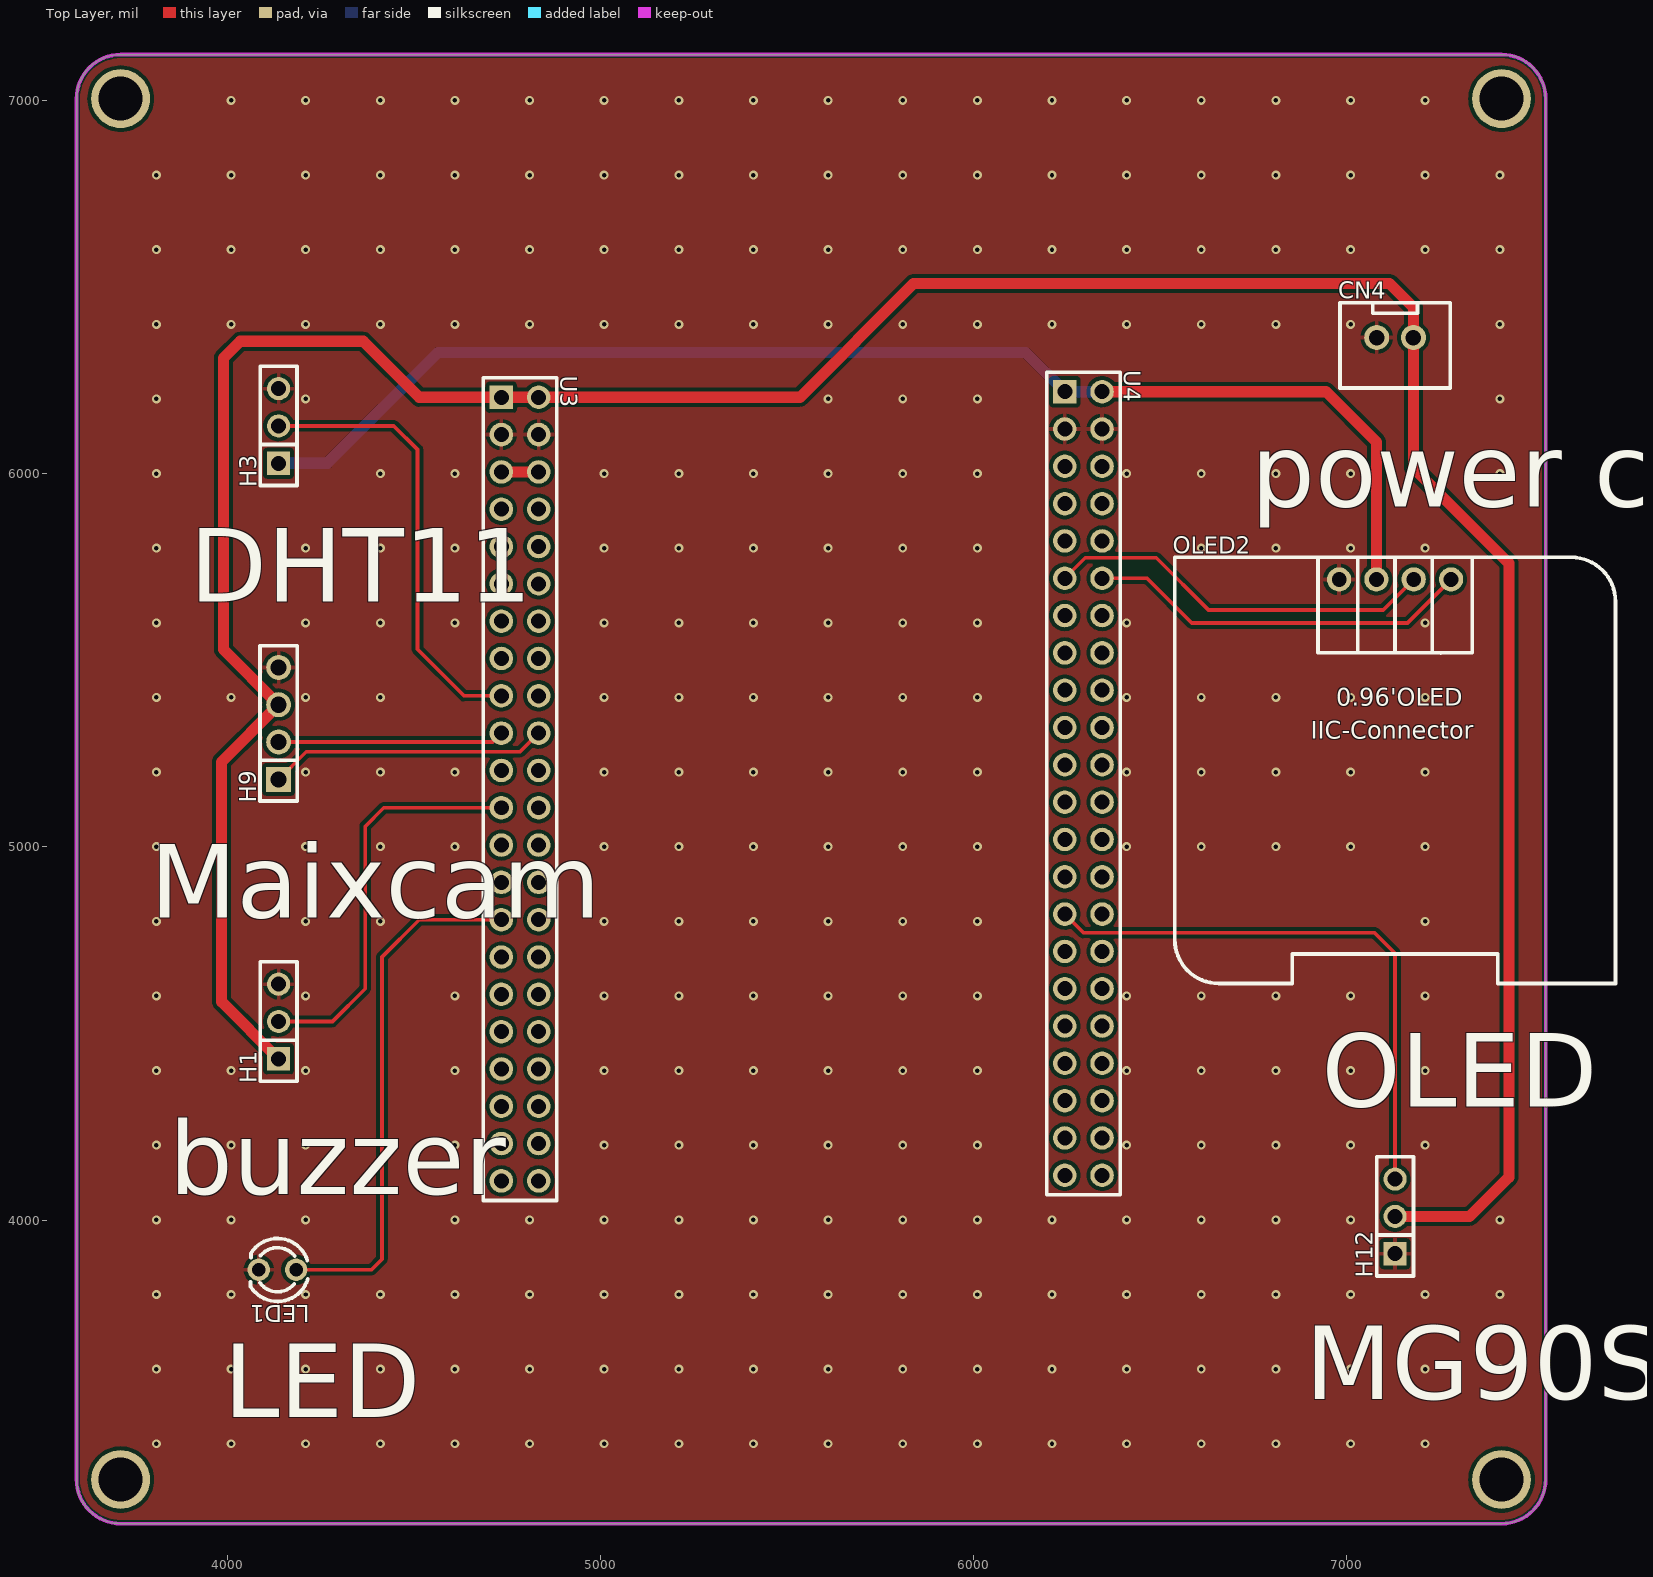
[diagram p0: Top Layer view]
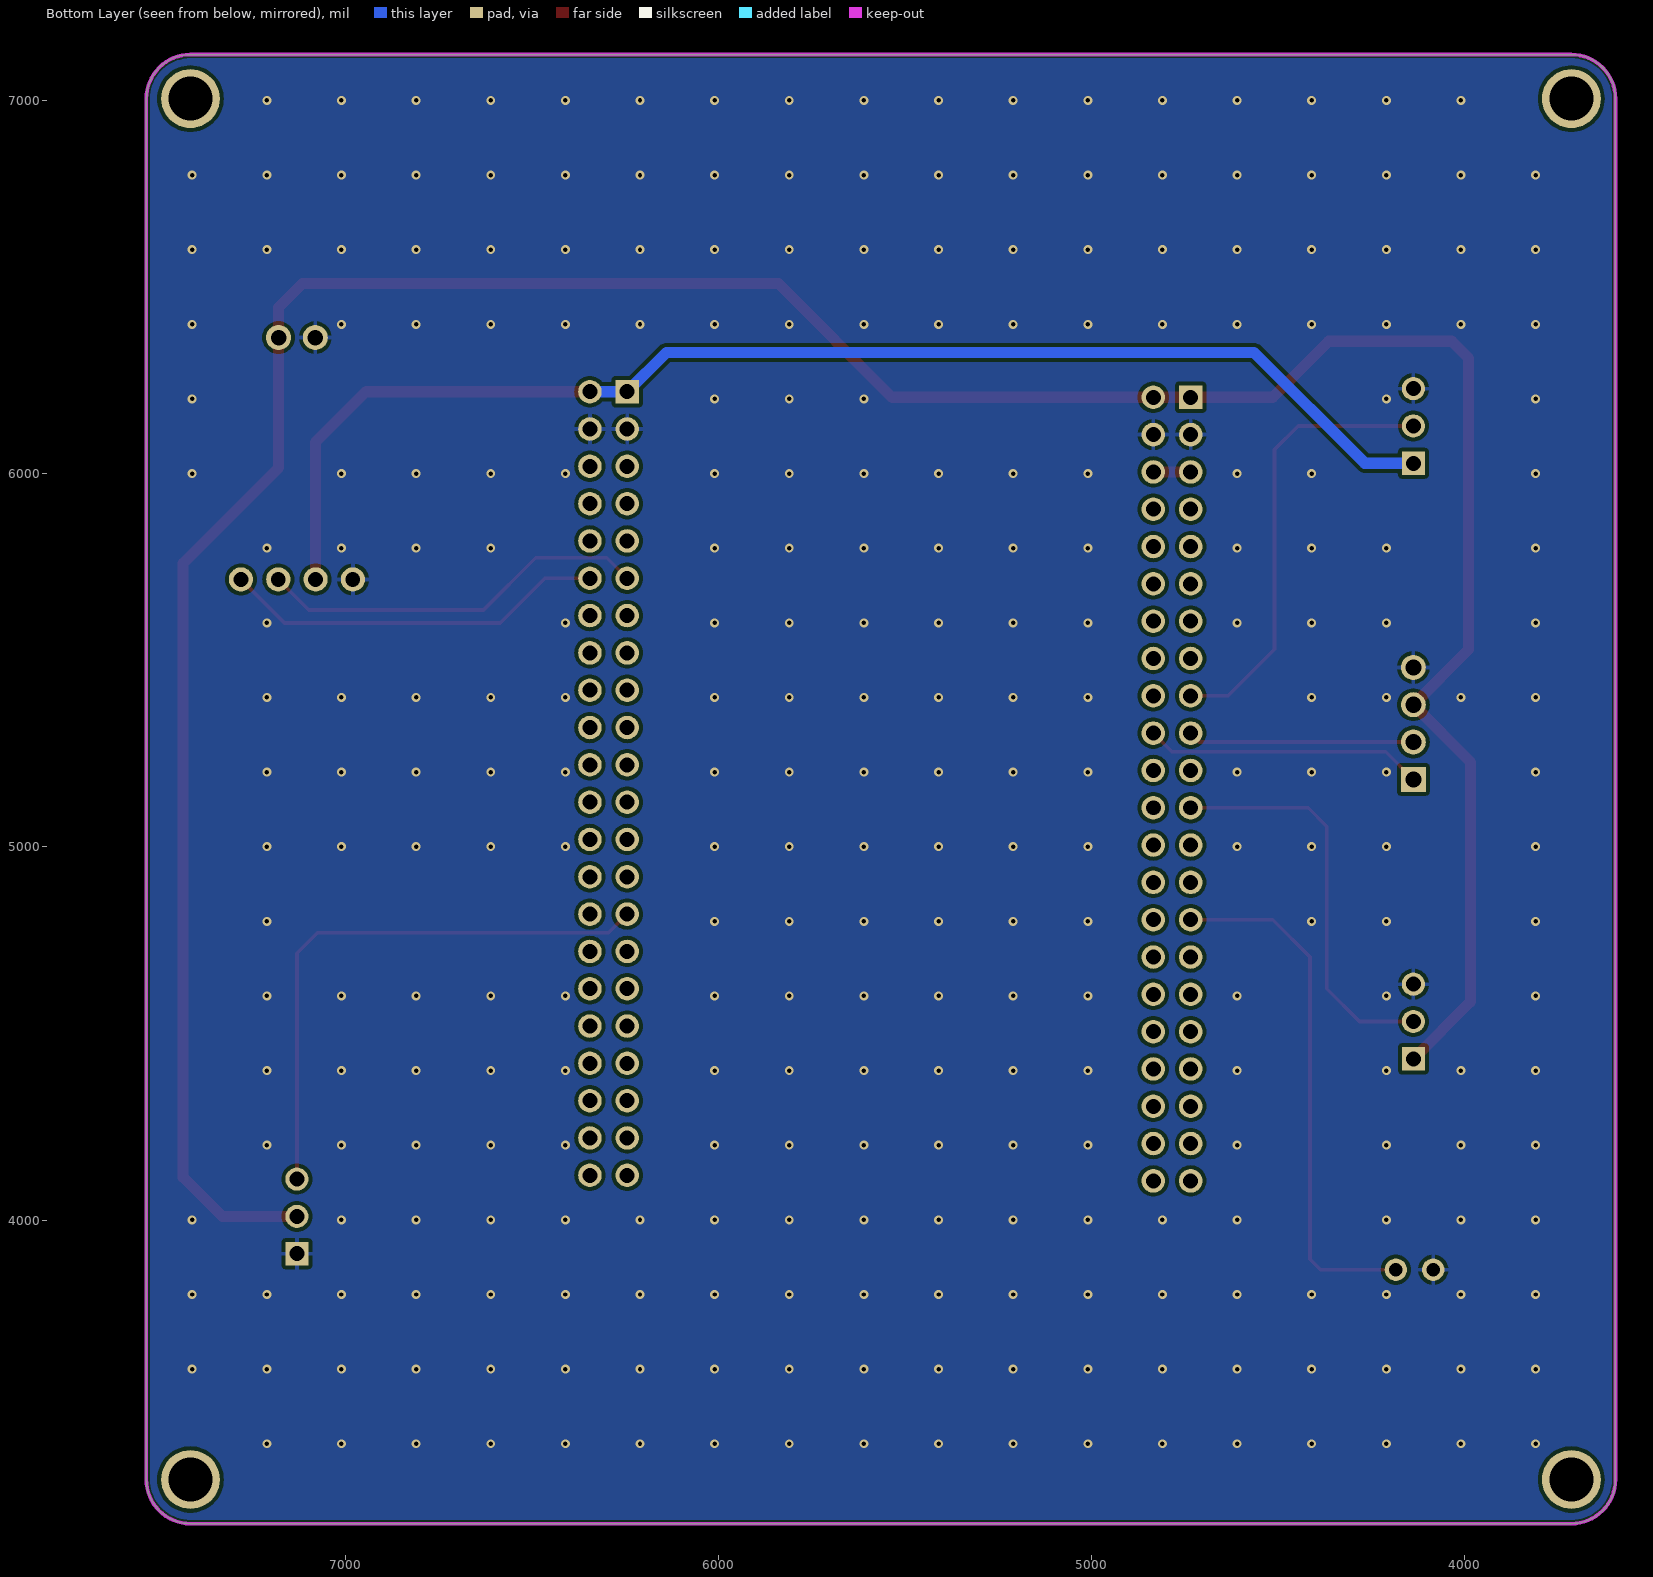
[diagram p1: Bottom Layer view, seen from below]
# Altium PCB MISC89054.pcbdoc
Units mil, origin at the board's own origin, x right, y up, seen from the top; angles counter-clockwise.
Board outline 3937.01 x 3937.01 mil, 2 copper layers (Top Layer, Bottom Layer), stack 62.206 mil thick; 9 components, 82 nets, 113 pads, 291 vias.

## Layer stack, top to bottom
Top Solder Mask Layer: solder mask 0.394, Dk 3.3
Top Layer: signal copper 1.379
Dielectric1: surface 59.449, FR4, Dk 4.5
Bottom Layer: signal copper 1.378
Bottom Solder Mask Layer: solder mask 0.394, Dk 3.3

## Board outline
3714.61,7123.5 ccw(c3714.61,7005.39) 3596.5,7005.39 3596.5,3304.61 ccw(c3714.61,3304.61) 3714.61,3186.5 7415.39,3186.5 ccw(c7415.39,3304.61) 7533.5,3304.61 7533.5,7005.39 ccw(c7415.39,7005.39) 7415.39,7123.5 3714.61,7123.5

## Design rules (kind name [scope] priority, off if disabled: settings)
BoardOutlineClearance copperThickness2oz_1 [All] p2 off: genericclearance=7.99 ignorepadtopadclearanceinfootprint=FALSE except(0: Arc-SplitContinuation Track-SplitContinuation SMDPad-SplitContinuation THPad-SplitContinuation Via-SplitContinuation Fill-SplitContinuation Region-SplitContinuation Poly-SplitContinuation Text-SplitContinuation Hole-SplitContinuation; 5.98: Arc-CutoutEdge Track-CutoutEdge SMDPad-CutoutEdge THPad-CutoutEdge Via-CutoutEdge Text-CutoutEdge; 6.9: Hole-OutlineEdge Hole-CutoutEdge; 10: Poly-OutlineEdge Poly-CutoutEdge; 11.81: Arc-OutlineEdge Track-OutlineEdge SMDPad-OutlineEdge THPad-OutlineEdge Via-OutlineEdge Fill-OutlineEdge Region-OutlineEdge Text-OutlineEdge Fill-CutoutEdge Region-CutoutEdge)
BoardOutlineClearance Plane_innerPlane_1 [All] p4 off: genericclearance=4.02 ignorepadtopadclearanceinfootprint=FALSE except(0: Arc-SplitContinuation Track-SplitContinuation SMDPad-SplitContinuation THPad-SplitContinuation Via-SplitContinuation Fill-SplitContinuation Region-SplitContinuation Poly-SplitContinuation Text-SplitContinuation Hole-SplitContinuation; 5.98: Arc-CutoutEdge Track-CutoutEdge SMDPad-CutoutEdge THPad-CutoutEdge Via-CutoutEdge Text-CutoutEdge; 6.9: Hole-OutlineEdge Hole-CutoutEdge; 10: Poly-OutlineEdge Poly-CutoutEdge; 11.81: Arc-OutlineEdge Track-OutlineEdge SMDPad-OutlineEdge THPad-OutlineEdge Via-OutlineEdge Fill-OutlineEdge Region-OutlineEdge Text-OutlineEdge Fill-CutoutEdge Region-CutoutEdge)
BoardOutlineClearance Copper_copperRegion_1 [All] p6 off: genericclearance=4.02 ignorepadtopadclearanceinfootprint=FALSE except(0: Arc-SplitContinuation Track-SplitContinuation SMDPad-SplitContinuation THPad-SplitContinuation Via-SplitContinuation Fill-SplitContinuation Region-SplitContinuation Poly-SplitContinuation Text-SplitContinuation Hole-SplitContinuation; 5.98: Arc-CutoutEdge Track-CutoutEdge SMDPad-CutoutEdge THPad-CutoutEdge Via-CutoutEdge Text-CutoutEdge; 6.9: Hole-OutlineEdge Hole-CutoutEdge; 10: Poly-OutlineEdge Poly-CutoutEdge; 11.81: Arc-OutlineEdge Track-OutlineEdge SMDPad-OutlineEdge THPad-OutlineEdge Via-OutlineEdge Fill-OutlineEdge Region-OutlineEdge Text-OutlineEdge Fill-CutoutEdge Region-CutoutEdge)
BoardOutlineClearance Copper_copperRegion_copperThickness1oz_1 [All] p8 off: genericclearance=4.02 ignorepadtopadclearanceinfootprint=FALSE except(0: Arc-SplitContinuation Track-SplitContinuation SMDPad-SplitContinuation THPad-SplitContinuation Via-SplitContinuation Fill-SplitContinuation Region-SplitContinuation Poly-SplitContinuation Text-SplitContinuation Hole-SplitContinuation; 5.98: Arc-CutoutEdge Track-CutoutEdge SMDPad-CutoutEdge THPad-CutoutEdge Via-CutoutEdge Text-CutoutEdge; 6.9: Hole-OutlineEdge Hole-CutoutEdge; 10: Poly-OutlineEdge Poly-CutoutEdge; 11.81: Arc-OutlineEdge Track-OutlineEdge SMDPad-OutlineEdge THPad-OutlineEdge Via-OutlineEdge Fill-OutlineEdge Region-OutlineEdge Text-OutlineEdge Fill-CutoutEdge Region-CutoutEdge)
BoardOutlineClearance Copper_copperRegion_Copper_copperRegion_1 [All] p10 off: genericclearance=4.02 ignorepadtopadclearanceinfootprint=FALSE except(0: Arc-SplitContinuation Track-SplitContinuation SMDPad-SplitContinuation THPad-SplitContinuation Via-SplitContinuation Fill-SplitContinuation Region-SplitContinuation Poly-SplitContinuation Text-SplitContinuation Hole-SplitContinuation; 5.98: Arc-CutoutEdge Track-CutoutEdge SMDPad-CutoutEdge THPad-CutoutEdge Via-CutoutEdge Text-CutoutEdge; 6.9: Hole-OutlineEdge Hole-CutoutEdge; 10: Poly-OutlineEdge Poly-CutoutEdge; 11.81: Arc-OutlineEdge Track-OutlineEdge SMDPad-OutlineEdge THPad-OutlineEdge Via-OutlineEdge Fill-OutlineEdge Region-OutlineEdge Text-OutlineEdge Fill-CutoutEdge Region-CutoutEdge)
BoardOutlineClearance copperThickness1oz_1 [All] p12: genericclearance=4.02 ignorepadtopadclearanceinfootprint=FALSE except(0: Arc-SplitContinuation Track-SplitContinuation SMDPad-SplitContinuation THPad-SplitContinuation Via-SplitContinuation Fill-SplitContinuation Region-SplitContinuation Poly-SplitContinuation Text-SplitContinuation Hole-SplitContinuation; 5.98: Arc-CutoutEdge Track-CutoutEdge SMDPad-CutoutEdge THPad-CutoutEdge Via-CutoutEdge Text-CutoutEdge; 6.9: Hole-OutlineEdge Hole-CutoutEdge; 10: Poly-OutlineEdge Poly-CutoutEdge; 11.81: Arc-OutlineEdge Track-OutlineEdge SMDPad-OutlineEdge THPad-OutlineEdge Via-OutlineEdge Fill-OutlineEdge Region-OutlineEdge Text-OutlineEdge Fill-CutoutEdge Region-CutoutEdge)
Clearance copperThickness2oz [All] p1 off: gap=7.99 ignorepadtopadclearanceinfootprint=FALSE except(5.98: SMDPad-Track SMDPad-SMDPad THPad-Track SMDPad-THPad THPad-THPad Track-Via SMDPad-Via THPad-Via Via-Via Fill-SMDPad Region-SMDPad Fill-THPad Region-THPad Fill-Via Region-Via Fill-Fill Fill-Region Region-Region Arc-Track Arc-SMDPad Arc-THPad Arc-Via Fill-Arc Region-Arc Arc-Arc Text-Track SMDPad-Text Text-THPad Text-Via Fill-Text Region-Text Arc-Text Text-Text; 6.9: Hole-Track Hole-SMDPad Hole-THPad Hole-Via Fill-Hole Region-Hole Hole-Arc Hole-Text; 10: Poly-Track Poly-SMDPad Poly-THPad Poly-Via Poly-Fill Poly-Region Poly-Poly Poly-Arc Poly-Text Poly-Hole; 11.81: Fill-Track Region-Track)
Clearance Plane_innerPlane [All] p3 off: gap=4.02 ignorepadtopadclearanceinfootprint=FALSE except(5.98: SMDPad-Track SMDPad-SMDPad THPad-Track SMDPad-THPad THPad-THPad Track-Via SMDPad-Via THPad-Via Via-Via Fill-SMDPad Region-SMDPad Fill-THPad Region-THPad Fill-Via Region-Via Fill-Fill Fill-Region Region-Region Arc-Track Arc-SMDPad Arc-THPad Arc-Via Fill-Arc Region-Arc Arc-Arc Text-Track SMDPad-Text Text-THPad Text-Via Fill-Text Region-Text Arc-Text Text-Text; 6.9: Hole-Track Hole-SMDPad Hole-THPad Hole-Via Fill-Hole Region-Hole Hole-Arc Hole-Text; 10: Poly-Track Poly-SMDPad Poly-THPad Poly-Via Poly-Fill Poly-Region Poly-Poly Poly-Arc Poly-Text Poly-Hole; 11.81: Fill-Track Region-Track)
Clearance Copper_copperRegion [All] p5 off: gap=4.02 ignorepadtopadclearanceinfootprint=FALSE except(5.98: SMDPad-Track SMDPad-SMDPad THPad-Track SMDPad-THPad THPad-THPad Track-Via SMDPad-Via THPad-Via Via-Via Fill-SMDPad Region-SMDPad Fill-THPad Region-THPad Fill-Via Region-Via Fill-Fill Fill-Region Region-Region Arc-Track Arc-SMDPad Arc-THPad Arc-Via Fill-Arc Region-Arc Arc-Arc Text-Track SMDPad-Text Text-THPad Text-Via Fill-Text Region-Text Arc-Text Text-Text; 6.9: Hole-Track Hole-SMDPad Hole-THPad Hole-Via Fill-Hole Region-Hole Hole-Arc Hole-Text; 10: Poly-Track Poly-SMDPad Poly-THPad Poly-Via Poly-Fill Poly-Region Poly-Poly Poly-Arc Poly-Text Poly-Hole; 11.81: Fill-Track Region-Track)
Clearance Copper_copperRegion_copperThickness1oz [All] p7 off: gap=4.02 ignorepadtopadclearanceinfootprint=FALSE except(5.98: SMDPad-Track SMDPad-SMDPad THPad-Track SMDPad-THPad THPad-THPad Track-Via SMDPad-Via THPad-Via Via-Via Fill-SMDPad Region-SMDPad Fill-THPad Region-THPad Fill-Via Region-Via Fill-Fill Fill-Region Region-Region Arc-Track Arc-SMDPad Arc-THPad Arc-Via Fill-Arc Region-Arc Arc-Arc Text-Track SMDPad-Text Text-THPad Text-Via Fill-Text Region-Text Arc-Text Text-Text; 6.9: Hole-Track Hole-SMDPad Hole-THPad Hole-Via Fill-Hole Region-Hole Hole-Arc Hole-Text; 10: Poly-Track Poly-SMDPad Poly-THPad Poly-Via Poly-Fill Poly-Region Poly-Poly Poly-Arc Poly-Text Poly-Hole; 11.81: Fill-Track Region-Track)
Clearance Copper_copperRegion_Copper_copperRegion [All] p9 off: gap=4.02 ignorepadtopadclearanceinfootprint=FALSE except(5.98: SMDPad-Track SMDPad-SMDPad THPad-Track SMDPad-THPad THPad-THPad Track-Via SMDPad-Via THPad-Via Via-Via Fill-SMDPad Region-SMDPad Fill-THPad Region-THPad Fill-Via Region-Via Fill-Fill Fill-Region Region-Region Arc-Track Arc-SMDPad Arc-THPad Arc-Via Fill-Arc Region-Arc Arc-Arc Text-Track SMDPad-Text Text-THPad Text-Via Fill-Text Region-Text Arc-Text Text-Text; 6.9: Hole-Track Hole-SMDPad Hole-THPad Hole-Via Fill-Hole Region-Hole Hole-Arc Hole-Text; 10: Poly-Track Poly-SMDPad Poly-THPad Poly-Via Poly-Fill Poly-Region Poly-Poly Poly-Arc Poly-Text Poly-Hole; 11.81: Fill-Track Region-Track)
Clearance copperThickness1oz [All] p11: gap=4.02 ignorepadtopadclearanceinfootprint=FALSE except(5.98: SMDPad-Track SMDPad-SMDPad THPad-Track SMDPad-THPad THPad-THPad Track-Via SMDPad-Via THPad-Via Via-Via Fill-SMDPad Region-SMDPad Fill-THPad Region-THPad Fill-Via Region-Via Fill-Fill Fill-Region Region-Region Arc-Track Arc-SMDPad Arc-THPad Arc-Via Fill-Arc Region-Arc Arc-Arc Text-Track SMDPad-Text Text-THPad Text-Via Fill-Text Region-Text Arc-Text Text-Text; 6.9: Hole-Track Hole-SMDPad Hole-THPad Hole-Via Fill-Hole Region-Hole Hole-Arc Hole-Text; 10: Poly-Track Poly-SMDPad Poly-THPad Poly-Via Poly-Fill Poly-Region Poly-Poly Poly-Arc Poly-Text Poly-Hole; 11.81: Fill-Track Region-Track)
DiffPairsRouting differentialPair [All] p1: maxlimit=6 minlimit=6 mostfreqgap=6 toplayer_minwidth=5 toplayer_prefwidth=10 toplayer_maxwidth=100 toplayer_mingap=6 toplayer_prefgap=6 toplayer_maxgap=6 bottomlayer_minwidth=5 bottomlayer_prefwidth=10 bottomlayer_maxwidth=100 bottomlayer_mingap=6 bottomlayer_prefgap=6 bottomlayer_maxgap=6 maxuncoupledlength=10
HoleToHoleClearance otherClearance [All] p1: gap=11.81 allowstackedmicrovias=TRUE
Length netLength [All] p1: minlimit=0 maxlimit=0
PasteMaskExpansion pasteMaskExpansion [All] p1: expansion=0
PlaneConnect innerPlane [All] p1: planeconnectstyle=Relief reliefexpansion=20 reliefentries=4 reliefconductorwidth=10 reliefairgap=10
PolygonConnect copperRegion_copperThickness1oz [All] p1 off: connectstyle=Relief reliefconductorwidth=10 reliefentries=4 polygonreliefangle="90 Angle" airgapwidth=10 via.connectstyle=Relief via.reliefconductorwidth=10 via.reliefentries=4 via.polygonreliefangle="90 Angle" via.airgapwidth=10
PolygonConnect copperRegion_Copper_copperRegion [All] p2 off: connectstyle=Relief reliefconductorwidth=10 reliefentries=4 polygonreliefangle="90 Angle" airgapwidth=10 via.connectstyle=Relief via.reliefconductorwidth=10 via.reliefentries=4 via.polygonreliefangle="90 Angle" via.airgapwidth=10
PolygonConnect copperRegion [All] p3: connectstyle=Relief reliefconductorwidth=10 reliefentries=4 polygonreliefangle="90 Angle" airgapwidth=10 via.connectstyle=Relief via.reliefconductorwidth=10 via.reliefentries=4 via.polygonreliefangle="90 Angle" via.airgapwidth=10
RoutingVias viaSize [All] p1: holewidth=12.01 width=24.02 viastyle="Through Hole" minholewidth=11.81 minwidth=19.68 maxholewidth=248.03 maxwidth=393.7
SolderMaskExpansion solderMaskExpansion [IsVia] p1: expansion=-1000 istentingtop=TRUE
SolderMaskExpansion solderMaskExpansion [All] p2: expansion=2 istentingtop=FALSE
Width copperThickness2oz_2 [All] p1 off: maxlimit=100 minlimit=8 preferedwidth=10
Width copperThickness1oz_2 [All] p2: maxlimit=100 minlimit=5 preferedwidth=10

## Components (designator, comment, footprint, x,y, rotation, side; value= is the part's Value field where it differs from the comment)
CN4 "XH2.54*2P_through-hole" CONN-TH_2P-P2.50-XH2.54-2P 7130,6365 r0 top
H1 "" HDR-TH_3P-P2.54-V-F 4138.13,4532.17 r90 top
H3 "" HDR-TH_3P-P2.54-V-F 4138.13,6128.19 r90 top
H9 "" HDR-TH_4P-P2.54-V-F 4138.13,5331.08 r90 top
H12 "" HDR-TH_3P-P2.54-V-F 7130,4009.81 r90 top
LED1 "" LED_TH-3mm 4135,3866.97 r180 top
OLED2 "" 0.96OLED_4P 7130,5716.87 r0 top
U3 "through-hole pin header_2.54_2*22" HDR-TH_44P-P2.54-V-M-R2-C22-S2.54 4785,5155 r270 top
U4 "through-hole pin header_2.54_2*22" HDR-TH_44P-P2.54-V-M-R2-C22-S2.54 6294.84,5170 r270 top

## Footprints (in the part's own frame and the unit in brackets; to place one, negate y for a bottom-side part, rotate by r counter-clockwise, add the part's x,y. Pads: shape width x height; smd on the part's side, far side on the other; paste and mask are expansions set on the pad)
0.96OLED_4P [mm]
  round 1.65 hole 1 copper offset 0,0: 1(-3.81,-0.001) 2(-1.27,0.002) 3(1.27,0.002) 4(3.81,0.002)
  silkscreen extent -15,-27.5 15,1.5
CONN-TH_2P-P2.50-XH2.54-2P [mm]
  round 1.7 hole 1.05 paste+0 mask+0.05: 1(1.25,0) 2(-1.25,0)
  silkscreen extent -3.75,-3.42 3.75,2.37
HDR-TH_3P-P2.54-V-F [mil]
  rect 62x62 hole 40.16: 1(-100,0)
  round 62 hole 40.16: 2(0,0) 3(100,0)
  silkscreen extent -160,-49 160,49
HDR-TH_4P-P2.54-V-F [mm]
  rect 1.7x1.7 hole 1.1: 1(-3.81,0)
  round 1.7 hole 1.1: 2(-1.27,0) 3(1.27,0) 4(3.81,0)
  silkscreen extent -5.29,-1.27 5.29,1.27
HDR-TH_44P-P2.54-V-M-R2-C22-S2.54 [mm]
  rect 1.6x1.6 hole 1.02 paste+0 mask+0.05: 1(-26.67,-1.27)
  round 1.6 hole 1.02 paste+0 mask+0.05: 2(-26.67,1.27) 3(-24.13,-1.27) 4(-24.13,1.27) 5(-21.59,-1.27) 6(-21.59,1.27) 7(-19.05,-1.27) 8(-19.05,1.27) 9(-16.51,-1.27) 10(-16.51,1.27) 11(-13.97,-1.27) 12(-13.97,1.27) 13(-11.43,-1.27) 14(-11.43,1.27) 15(-8.89,-1.27) 16(-8.89,1.27) 17(-6.35,-1.27) 18(-6.35,1.27) 19(-3.81,-1.27) 20(-3.81,1.27) 21(-1.27,-1.27) 22(-1.27,1.27) 23(1.27,-1.27) 24(1.27,1.27) 25(3.81,-1.27) 26(3.81,1.27) 27(6.35,-1.27) 28(6.35,1.27) 29(8.89,-1.27) 30(8.89,1.27) 31(11.43,-1.27) 32(11.43,1.27) 33(13.97,-1.27) 34(13.97,1.27) 35(16.51,-1.27) 36(16.51,1.27) 37(19.05,-1.27) 38(19.05,1.27) 39(21.59,-1.27) 40(21.59,1.27) 41(24.13,-1.27) 42(24.13,1.27) 43(26.67,-1.27) 44(26.67,1.27)
  silkscreen extent -28,-2.5 28,2.5
LED_TH-3mm [mil]
  round 60 hole 36 paste+0 mask+2: 1(-50,0) 2(50,0)
  silkscreen extent -81,-84 72,85

## Free pads (board coordinates)
  round 157.48 hole 118.11: 1(3714.61,7005.39) 1(3714.61,3304.61) 1(7415.39,7005.39) 1(7415.39,3304.61)

## Via types
v1: diameter 24.02, hole 12, Top Layer to Bottom Layer, 291 vias

## Nets (pads, with @x,y where several pads share a name; then routed paths per layer and width w, separated by ;. In a path a pad name is that pad's centre, name@x,y a point inside that pad or via, vN(x,y) a via of type N, cw(c..) or ccw(c..) an arc to the next point about the centre after c; other vN are vias at no path point)
+5V: CN4.1 H1.1 H9.3 H12.2 U3.1 U3.2 | length 8274.3
  Top Layer w30: H1.1 3985,4585.3 3985,5227.94 H9.3 3990,5529.21 3990,6310 4035,6355 4365,6355 4515,6205 U3.1 U3.2 5535,6205 5840,6510 7115,6510 7179.21,6445.79 CN4.1 7179.21,6015.79 7435,5760 7435,4115 7329.81,4009.81 H12.2
A0: H3.2 U3.17 | length 1209.8
  Top Layer w10: H3.2 4446.81,6128.19 4510,6065 4510,5530 4635,5405 U3.17
A1: U3.18
A2: H9.2 U3.19 | length 606.8
  Top Layer w10: H9.2 4711.07,5281.08 U3.19
A3: H9.1 U3.20 | length 748.2
  Top Layer w10: H9.1 4212.06,5255 4785,5255 U3.20
A4: U3.21
A5: U3.22
A6: H1.2 U3.23 | length 1089
  Top Layer w10: H1.2 4282.17,4532.17 4370,4620 4370,5055 4420,5105 U3.23
A7: U3.24
A8: H12.3 U4.29 | length 1533.8
  Top Layer w10: U4.29 6294.85,4770 7075,4770 7130,4715 H12.3
A9: U4.31
A10: U4.32
A11: U4.30
A12: U4.27
A15: U4.28
B0: U3.27
B1: U3.28
B2: LED1.1 U3.29 | length 1413
  Top Layer w10: LED1.1 4386.97,3866.97 4415,3895 4415,4705 4515,4805 U3.29
B3: U4.16
B4: U4.13
B5: U4.14
B6: OLED2.3 U4.11 | length 1049.9
  Top Layer w10: U4.11 6299.84,5775 6490,5775 6630,5635 7098.08,5635 OLED2.3
B7: OLED2.4 U4.12 | length 1033.3
  Top Layer w10: U4.12 6465,5720 6585,5600 7163.08,5600 OLED2.4
B8: U4.9
B9: U4.10
B10: U3.39
B11: U3.40
B12: U3.41
B13: U3.42
B14: U3.43
B15: U3.44
BOOT0: U4.5
BOOT1: U4.6
C0: U3.13
C1: U3.14
C2: U3.15
C3: U3.16
C4: U3.25
C5: U3.26
C6: U4.35
C7: U4.36
C8: U4.33
C9: U4.34
C10: U4.25
C11: U4.26
C12: U4.23
C13: U3.12
D0: U4.24
D1: U4.21
D2: U4.22
D3: U4.19
D4: U4.20
D5: U4.17
D6: U4.18
D7: U4.15
D8: U4.43
D9: U4.44
D10: U4.41
D11: U4.42
D12: U4.39
D13: U4.40
D14: U4.37
D15: U4.38
E0: U4.7
E1: U4.8
E2: U3.7
E3: U3.8
E4: U3.9
E5: U3.10
E6: U3.11
E7: U3.30
E8: U3.31
E9: U3.32
E10: U3.33
E11: U3.34
E12: U3.35
E13: U3.36
E14: U3.37
E15: U3.38
GND: CN4.2 H1.3 H3.3 H9.4 H12.1 LED1.2 OLED2.1 U3.3 U3.4 U4.3 U4.4
  other v1: 3810.6,3400.6 4010.6,3400.6 4210.6,3400.6 4410.6,3400.6 4610.6,3400.6 4810.6,3400.6 5010.6,3400.6 5210.6,3400.6 5410.6,3400.6 5610.6,3400.6 5810.6,3400.6 6010.6,3400.6 6210.6,3400.6 6410.6,3400.6 6610.6,3400.6 6810.6,3400.6 7010.6,3400.6 7210.6,3400.6 3810.6,3600.6 4010.6,3600.6 4210.6,3600.6 4410.6,3600.6 4610.6,3600.6 4810.6,3600.6 5010.6,3600.6 5210.6,3600.6 5410.6,3600.6 5610.6,3600.6 5810.6,3600.6 6010.6,3600.6 6210.6,3600.6 6410.6,3600.6 6610.6,3600.6 6810.6,3600.6 7010.6,3600.6 7210.6,3600.6 7410.6,3600.6 3810.6,3800.6 4010.6,3800.6 4210.6,3800.6 4410.6,3800.6 4610.6,3800.6 4810.6,3800.6 5010.6,3800.6 5210.6,3800.6 5410.6,3800.6 5610.6,3800.6 5810.6,3800.6 6010.6,3800.6 6210.6,3800.6 6410.6,3800.6 6610.6,3800.6 6810.6,3800.6 7010.6,3800.6 7210.6,3800.6 7410.6,3800.6 3810.6,4000.6 4010.6,4000.6 4210.6,4000.6 4610.6,4000.6 4810.6,4000.6 5010.6,4000.6 5210.6,4000.6 5410.6,4000.6 5610.6,4000.6 5810.6,4000.6 6010.6,4000.6 6210.6,4000.6 6410.6,4000.6 6610.6,4000.6 6810.6,4000.6 7010.6,4000.6 7410.6,4000.6 3810.6,4200.6 4010.6,4200.6 4210.6,4200.6 4610.6,4200.6 5010.6,4200.6 5210.6,4200.6 5410.6,4200.6 5610.6,4200.6 5810.6,4200.6 6010.6,4200.6 6410.6,4200.6 6610.6,4200.6 6810.6,4200.6 7010.6,4200.6 7210.6,4200.6 3810.6,4400.6 4010.6,4400.6 4210.6,4400.6 4610.6,4400.6 5010.6,4400.6 5210.6,4400.6 5410.6,4400.6 5610.6,4400.6 5810.6,4400.6 6010.6,4400.6 6410.6,4400.6 6610.6,4400.6 6810.6,4400.6 7010.6,4400.6 7210.6,4400.6 3810.6,4600.6 4210.6,4600.6 4610.6,4600.6 5010.6,4600.6 5210.6,4600.6 5410.6,4600.6 5610.6,4600.6 5810.6,4600.6 6010.6,4600.6 6410.6,4600.6 6610.6,4600.6 6810.6,4600.6 7010.6,4600.6 7210.6,4600.6 3810.6,4800.6 4210.6,4800.6 4410.6,4800.6 5010.6,4800.6 5210.6,4800.6 5410.6,4800.6 5610.6,4800.6 5810.6,4800.6 6010.6,4800.6 7210.6,4800.6 3810.6,5000.6 4210.6,5000.6 4410.6,5000.6 4610.6,5000.6 5010.6,5000.6 5210.6,5000.6 5410.6,5000.6 5610.6,5000.6 5810.6,5000.6 6010.6,5000.6 6410.6,5000.6 6610.6,5000.6 6810.6,5000.6 7010.6,5000.6 7210.6,5000.6 3810.6,5200.6 4210.6,5200.6 4410.6,5200.6 4610.6,5200.6 5010.6,5200.6 5210.6,5200.6 5410.6,5200.6 5610.6,5200.6 5810.6,5200.6 6010.6,5200.6 6410.6,5200.6 6610.6,5200.6 6810.6,5200.6 7010.6,5200.6 7210.6,5200.6 3810.6,5400.6 4010.6,5400.6 4210.6,5400.6 4410.6,5400.6 5010.6,5400.6 5210.6,5400.6 5410.6,5400.6 5610.6,5400.6 5810.6,5400.6 6010.6,5400.6 6410.6,5400.6 6610.6,5400.6 6810.6,5400.6 7010.6,5400.6 7210.6,5400.6 3810.6,5600.6 4210.6,5600.6 4410.6,5600.6 4610.6,5600.6 5010.6,5600.6 5210.6,5600.6 5410.6,5600.6 5610.6,5600.6 5810.6,5600.6 6010.6,5600.6 6410.6,5600.6 7210.6,5600.6 3810.6,5800.6 4210.6,5800.6 4410.6,5800.6 4610.6,5800.6 5010.6,5800.6 5210.6,5800.6 5410.6,5800.6 5610.6,5800.6 5810.6,5800.6 6010.6,5800.6 6610.6,5800.6 6810.6,5800.6 7010.6,5800.6 7210.6,5800.6 3810.6,6000.6 4410.6,6000.6 4610.6,6000.6 5010.6,6000.6 5210.6,6000.6 5410.6,6000.6 5610.6,6000.6 5810.6,6000.6 6010.6,6000.6 6410.6,6000.6 6610.6,6000.6 6810.6,6000.6 7010.6,6000.6 7410.6,6000.6 3810.6,6200.6 4210.6,6200.6 5610.6,6200.6 5810.6,6200.6 6010.6,6200.6 7410.6,6200.6 3810.6,6400.6 4010.6,6400.6 4210.6,6400.6 4410.6,6400.6 4610.6,6400.6 4810.6,6400.6 5010.6,6400.6 5210.6,6400.6 5410.6,6400.6 5610.6,6400.6 5810.6,6400.6 6010.6,6400.6 6210.6,6400.6 6410.6,6400.6 6610.6,6400.6 6810.6,6400.6 7010.6,6400.6 7410.6,6400.6 3810.6,6600.6 4010.6,6600.6 4210.6,6600.6 4410.6,6600.6 4610.6,6600.6 4810.6,6600.6 5010.6,6600.6 5210.6,6600.6 5410.6,6600.6 5610.6,6600.6 5810.6,6600.6 6010.6,6600.6 6210.6,6600.6 6410.6,6600.6 6610.6,6600.6 6810.6,6600.6 7010.6,6600.6 7210.6,6600.6 7410.6,6600.6 3810.6,6800.6 4010.6,6800.6 4210.6,6800.6 4410.6,6800.6 4610.6,6800.6 4810.6,6800.6 5010.6,6800.6 5210.6,6800.6 5410.6,6800.6 5610.6,6800.6 5810.6,6800.6 6010.6,6800.6 6210.6,6800.6 6410.6,6800.6 6610.6,6800.6 6810.6,6800.6 7010.6,6800.6 7210.6,6800.6 7410.6,6800.6 4010.6,7000.6 4210.6,7000.6 4410.6,7000.6 4610.6,7000.6 4810.6,7000.6 5010.6,7000.6 5210.6,7000.6 5410.6,7000.6 5610.6,7000.6 5810.6,7000.6 6010.6,7000.6 6210.6,7000.6 6410.6,7000.6 6610.6,7000.6 6810.6,7000.6 7010.6,7000.6 7210.6,7000.6
RESERT: U3.5 U3.6 | length 100
  Top Layer w30: U3.5 U3.6
VCC: H3.1 OLED2.2 U4.1 U4.2 | length 3532.3
  Top Layer w30: U4.2 6945,6220 7080,6085 OLED2.2
  Bottom Layer w30: H3.1 4268.19,6028.19 4565,6325 6139.85,6325 U4.1 U4.2

## Polygon pours and split planes (outlines as drawn)
GND on Bottom Layer (solid, remove dead copper, pour order 2): 3525,7245 3525,3080 7700,3080 7700,7245
GND on Top Layer (solid, remove dead copper, pour order 2): 3000,7415 3000,3000 7930,3000 7930,7415

## Keep-outs
Board Outline Layer:
  the board outline again, w10

## Silkscreen, mask and mechanical layers (free items; w line width, h text height)
Top Silkscreen Layer:
  text "power connector" at 6744.65,5911.53 h196.85
  text "DHT11" at 3899.53,5656.46 h196.85
  text "Maixcam" at 3793.35,4809.73 h196.85
  text "OLED" at 6933.44,4304.26 h196.85
  text "buzzer" at 3844.94,4069.69 h196.85
  text "MG90S" at 6888.85,3520 h196.85
  text "LED" at 3991.09,3471.57 h196.85